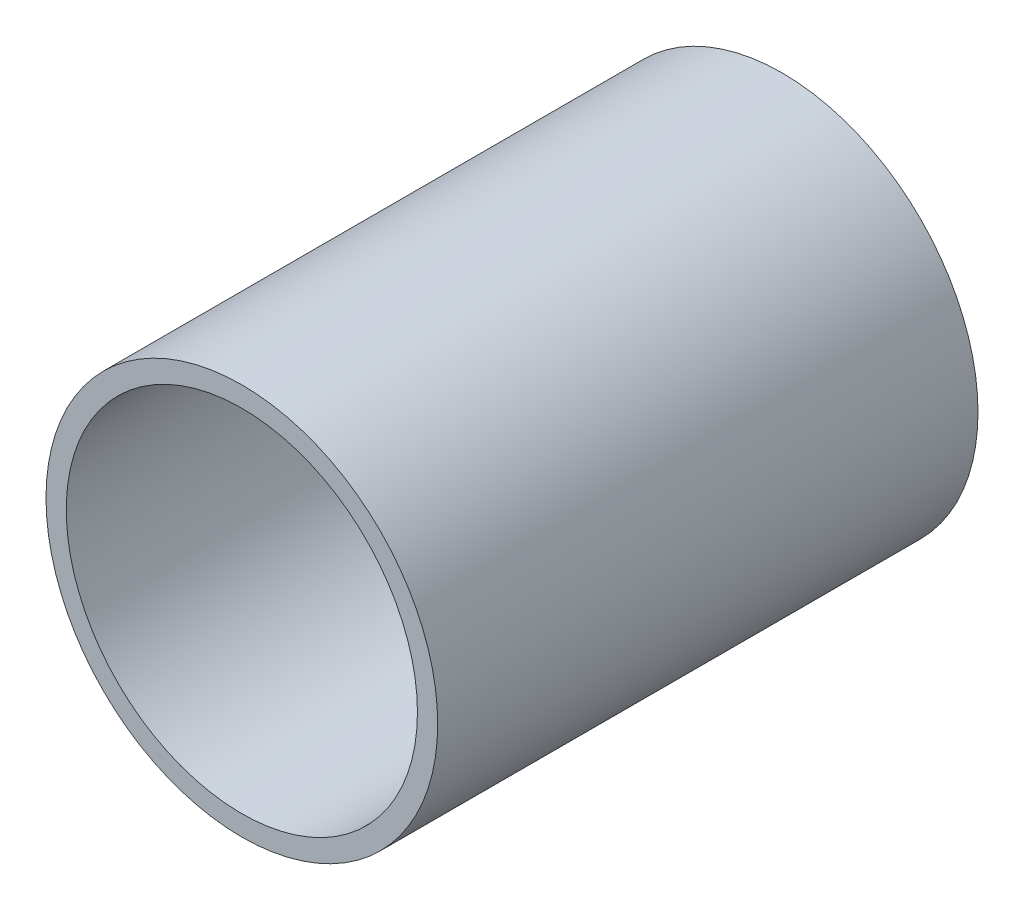
from build123d import *

# Parameters (mm, degrees)
SKETCH1_R           = 3.683
SKETCH1_R_2         = 3.302
BOSS_EXTRUDE1_DEPTH = 10.16
SCALE1_SCALE        = 2


with BuildPart() as part:
    # Sketch1 → Boss-Extrude1 (new body)
    with BuildSketch(Plane.XY):
        Circle(SKETCH1_R)
        Circle(SKETCH1_R_2, mode=Mode.SUBTRACT)
    extrude(amount=BOSS_EXTRUDE1_DEPTH)


with BuildPart() as part_1:
    # Scale1: scaled about (0, 0, 0)
    add(part.part.scale(SCALE1_SCALE))


solid = part_1.part
